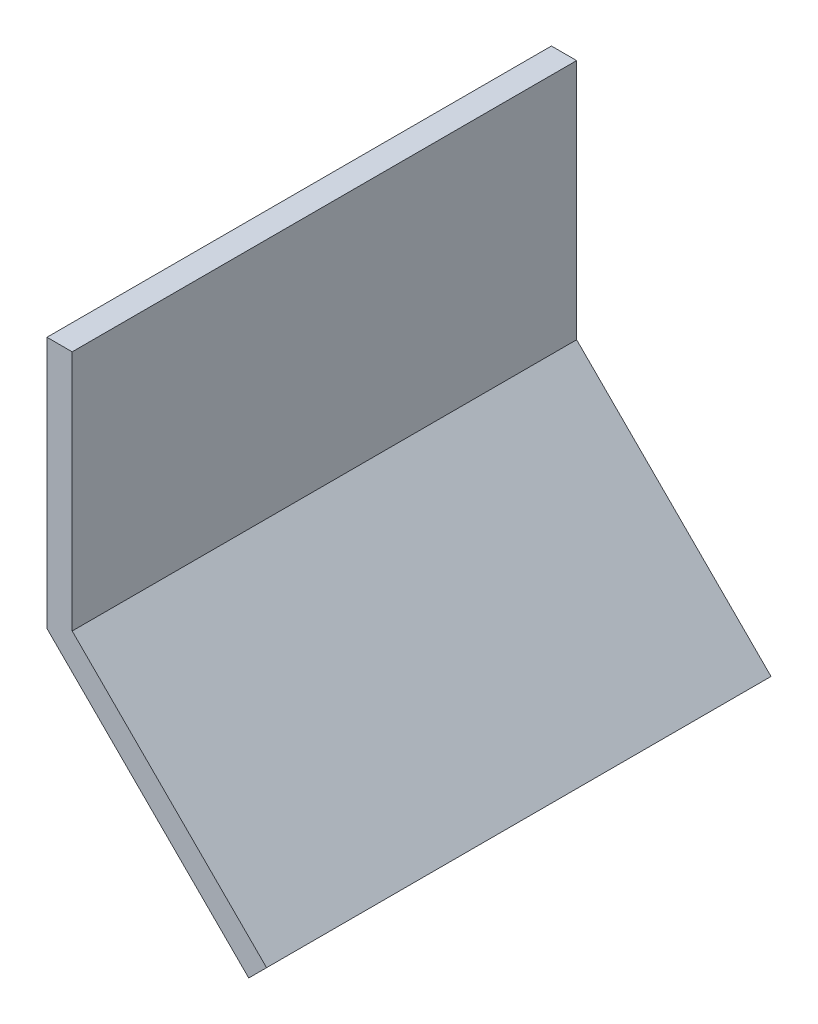
SolidWorks part; units mm, degrees
ref_plane "前视基准面" through (0, 0, 0) normal (0, 0, 1) x (1, 0, 0)
ref_plane "上视基准面" through (0, 0, 0) normal (0, 1, 0) x (1, 0, 0)
ref_plane "右视基准面" through (0, 0, 0) normal (1, 0, 0) x (0, 0, -1)
sketch "草图1" plane through (0, 0, 0) normal (0, 0, 1) x (1, 0, 0)
  line L0 (0, 0) -> (0, -50)
  line L1 (5, 0) -> (5, -47.9289)
  line L2 (5, -47.9289) -> (43.5355, -86.4645)
  line L3 (0, 0) -> (5, 0)
  line L4 (40, -90) -> (43.5355, -86.4645)
  line L6 (0, -50) -> (40, -90)
  dimension "D1" = 5
extrude "凸台-拉伸2" add sketch "草图1" along normal blind 100
sketch "草图2" plane through (5, 0, 0) normal (1, 0, 0) x (0, 0, -1)
  line L4 (-95, 0) -> (-95, -5)
  line L5 (-100, 0) -> (0, 0) construction
  line L6 (-95, -42.9289) -> (-95, -90)
  line L7 (-100, -90) -> (0, -90) construction
  line L8 (-5, -42.9289) -> (-5, -5)
  line L9 (-5, -5) -> (-95, -5)
  line L10 (-95, -5) -> (-95, -42.9289)
  line L11 (-95, -42.9289) -> (-5, -42.9289)
  line L12 (-5, -42.9289) -> (-5, -5)
  line L13 (-5, 0) -> (-5, -90)
  line L14 (-95, -5) -> (-95, -42.9289)
  line L15 (-5, -90) -> (0, -90)
  line L16 (0, -90) -> (0, 0)
  line L17 (-5, 0) -> (0, 0)
  line L18 (-95, 0) -> (-100, 0)
  line L19 (-100, 0) -> (-100, -90)
  line L20 (-100, -90) -> (-95, -90)
  line M5 (0, -47.9289) -> (0, 0)
  line M6 (0, 0) -> (-100, 0)
  line M7 (-100, 0) -> (-100, -47.9289)
  line M8 (-100, -47.9289) -> (0, -47.9289)
  dimension "D1" = 5
extrude "切除-拉伸1" cut sketch "草图2" against normal through all both and the other way through all contours L13 L12 M6 M8 M5 | L15 L16 L13 M8 | L19 L20 L6 M8 | L14 L4 L6 M6 M7 M8
sketch "草图3" plane through (0, 0, 95) normal (0, 0, 1) x (1, 0, 0)
  line L12 (0, -50) -> (40, -90)
  line L13 (40, -90) -> (43.5355, -86.4645)
  line L14 (43.5355, -86.4645) -> (5, -47.9289)
  line L15 (5, -47.9289) -> (5, 0)
  line L16 (5, 0) -> (0, 0)
  line L17 (0, 0) -> (0, -50)
  line L18 (0, -50) -> (40, -90)
  line L19 (40, -90) -> (43.5355, -86.4645)
  line L20 (43.5355, -86.4645) -> (5, -47.9289)
  line L21 (5, -47.9289) -> (5, 0)
  line L22 (5, 0) -> (0, 0)
  line L23 (0, 0) -> (0, -50)
  dimension "D1" = 0
extrude "凸台-拉伸3" add sketch "草图3" along normal blind 10
